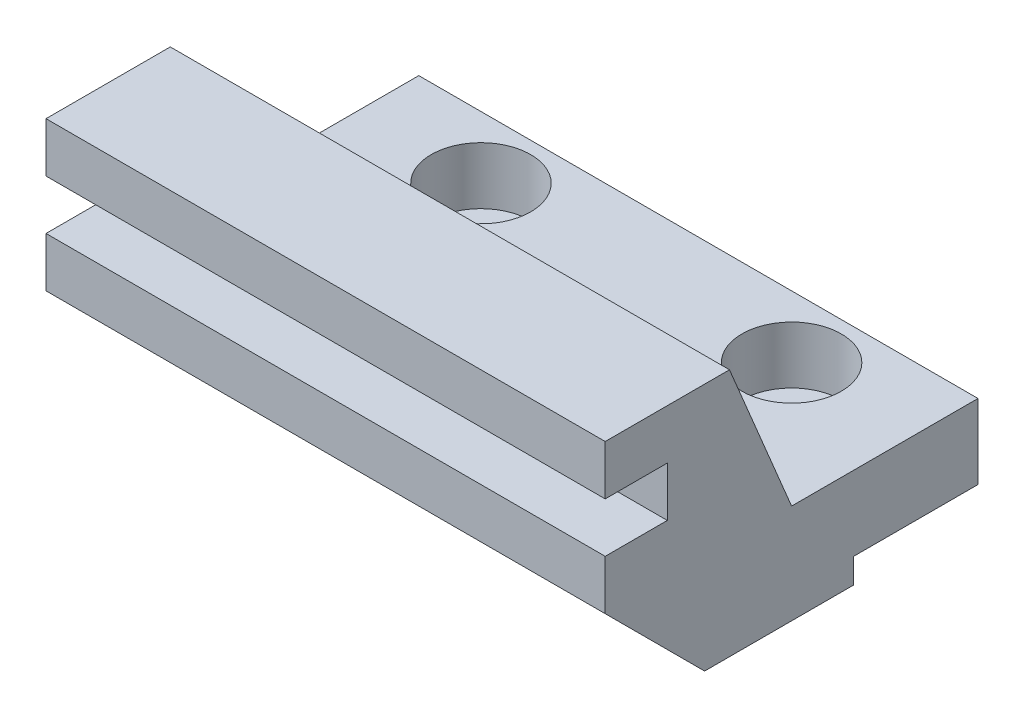
SolidWorks part; units mm, degrees
ref_plane "Front Plane" through (0, 0, 0) normal (0, 0, 1) x (1, 0, 0)
ref_plane "Top Plane" through (0, 0, 0) normal (0, 1, 0) x (1, 0, 0)
ref_plane "Right Plane" through (0, 0, 0) normal (1, 0, 0) x (0, 0, -1)
sketch "Sketch1" plane through (0, 0, 0) normal (0, 0, 1) x (1, 0, 0)
  line L1 (-22.5, 10) -> (22.5, 10)
  line L2 (-22.5, 10) -> (-22.5, -10)
  line L3 (-22.5, -10) -> (22.5, -10)
  line L4 (22.5, 10) -> (22.5, -10)
  line L5 (-22.5, 10) -> (22.5, -10) construction
  line L6 (-22.5, -10) -> (22.5, 10) construction
  point P0 (0, 0)
  dimension "D1" = 45
  dimension "D2" = 20
extrude "Boss-Extrude1" add sketch "Sketch1" along normal blind 30
sketch "Sketch2" plane through (-22.5, 0, 0) normal (-1, 0, 0) x (0, 0, 1)
  line L0 (30, 10) -> (30, -10) construction
  line L1 (0, -2) -> (15, -2)
  line L2 (30, 6) -> (25, 6)
  line L3 (30, 6) -> (30, 2)
  line L4 (30, 2) -> (25, 2)
  line L5 (25, 6) -> (25, 2)
  line L6 (30, 10) -> (0, 10) construction
  line L11 (0, 10) -> (0, -10) construction
  line L12 (15, -2) -> (20, 10)
  line L13 (20, 10) -> (0, 10)
  line L14 (0, 10) -> (0, -2)
  dimension "D1" = 4
  dimension "D2" = 5
  dimension "D3" = 4
  dimension "D4" = 12
  dimension "D5" = 15
  dimension "D6" = 20
extrude "Cut-Extrude1" cut sketch "Sketch2" against normal through all both and the other way through all
chamfer "Chamfer1" distance 8 angle 45 1 edges at (0, -10, 30)
hole_wizard "Hole for socket head cap screw, type1" positions "Sketch5" profile "Sketch6" counterbore size "M4" standard "GB" end condition through all
sketch "Sketch5" plane through (0, -2, 0) normal (0, 1, 0) x (1, 0, 0)
  line L0 (0, 0) -> (0, -7.1023) construction
  line L1 (22.5, 0) -> (-22.5, 0) construction
  point P0 (-12.5, -5)
  point P2 (12.5, -5)
  dimension "D1" = 25
  dimension "D2" = 5
sketch "Sketch6" plane through (-12.5, -2, 5) normal (1, 0, 0) x (0, 0, 1)
  line L0 (0, 0) -> (0, 8)
  line L1 (0, 8) -> (2.25, 8)
  line L3 (2.25, 8) -> (2.25, 4.6)
  line L4 (2.25, 4.6) -> (4, 4.6)
  line L5 (4, 4.6) -> (4, 0)
  line L7 (4, 0) -> (0, 0)
  line L11 (0, -6.35) -> (0, 107.95) construction
  dimension "通孔孔直径" = 4.5
  dimension "通孔孔深度" = 8
  dimension "柱形沉头孔直径" = 8
  dimension "柱形沉头孔深度" = 4.6
sketch "Sketch7" plane through (-22.5, 0, 0) normal (-1, 0, 0) x (0, 0, 1)
  line L0 (0, -2) -> (0, -10) construction
  line L1 (0, -8) -> (10, -8)
  line L2 (0, -8) -> (0, -10)
  line L3 (0, -10) -> (10, -10)
  line L4 (10, -8) -> (10, -10)
  line L5 (22, -10) -> (0, -10) construction
  dimension "D1" = 10
  dimension "D2" = 2
extrude "Cut-Extrude2" cut sketch "Sketch7" against normal through all both and the other way through all
